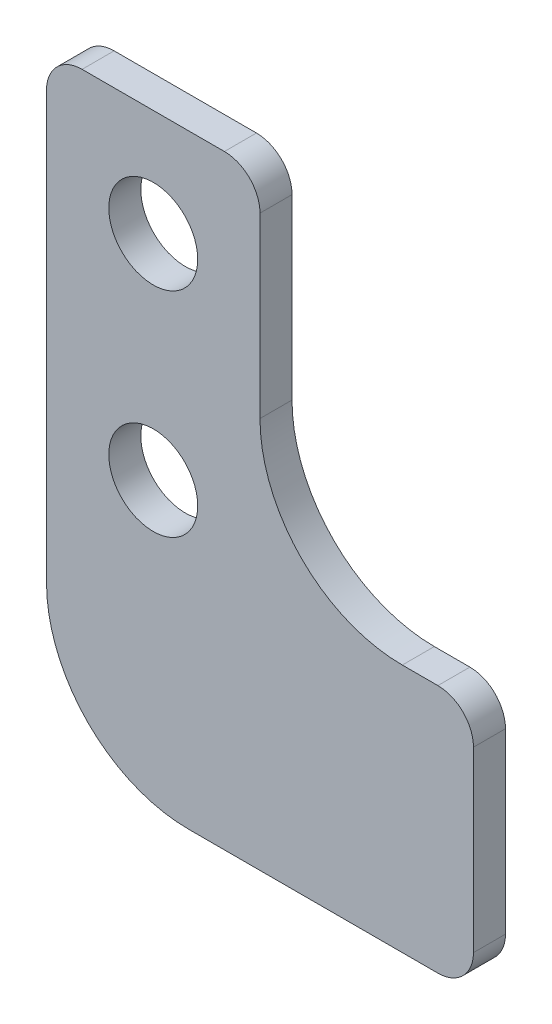
from build123d import *

# Parameters (mm, degrees)
SKETCH1_R           = 6.25
BOSS_EXTRUDE1_DEPTH = 4.5


with BuildPart() as part:
    # Sketch1 → Boss-Extrude1 (new body)
    with BuildSketch(Plane.XY):
        with BuildLine():
            Line((25, 85), (5, 85))
            ThreePointArc((5, 85), (1.464466094, 83.535533906), (0, 80))
            Line((0, 80), (0, 20))
            ThreePointArc((0, 20), (5.857864376, 5.857864376), (20, 0))
            Line((20, 0), (55, 0))
            ThreePointArc((55, 0), (58.535533906, 1.464466094), (60, 5))
            Line((60, 5), (60, 30))
            ThreePointArc((60, 30), (58.535533906, 33.535533906), (55, 35))
            Line((55, 35), (50, 35))
            ThreePointArc((50, 35), (35.857864376, 40.857864376), (30, 55))
            Line((30, 55), (30, 80))
            ThreePointArc((30, 80), (28.535533906, 83.535533906), (25, 85))
        make_face()
        with Locations((15, 40)):
            Circle(SKETCH1_R, mode=Mode.SUBTRACT)
        with Locations((15, 70)):
            Circle(SKETCH1_R, mode=Mode.SUBTRACT)
    extrude(amount=BOSS_EXTRUDE1_DEPTH)


solid = part.part
